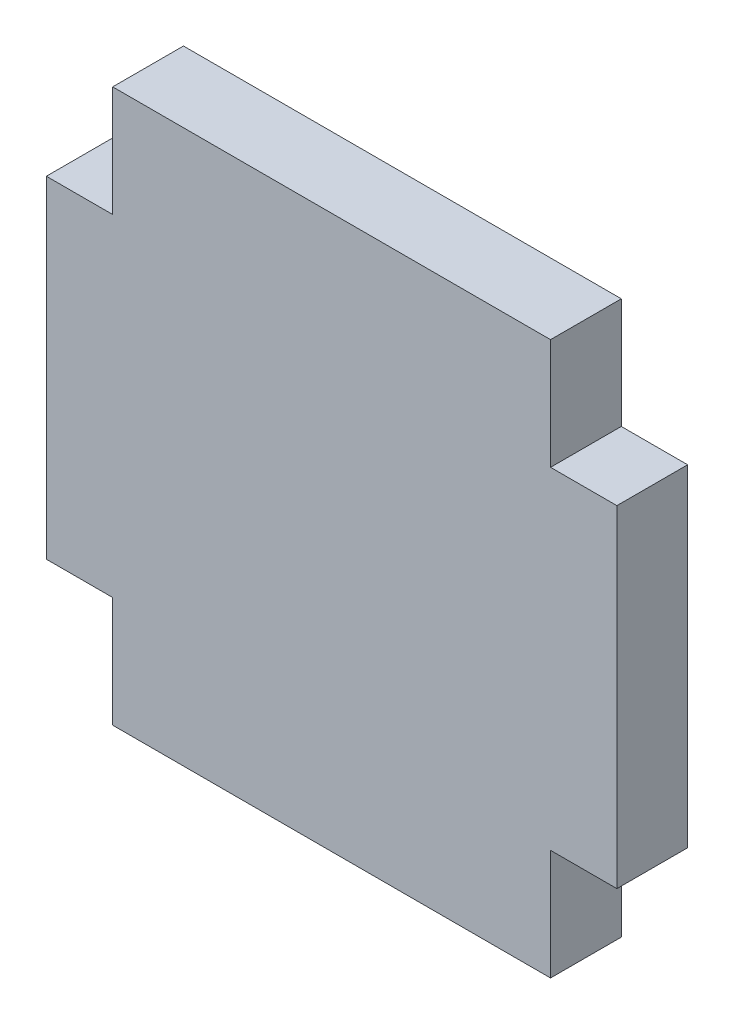
from build123d import *

# Parameters (mm, degrees)
BOSS_EXTRUDE1_DEPTH = 1.6


with BuildPart() as part:
    # Sketch1 → Boss-Extrude1 (new, symmetric)
    with BuildSketch(Plane.XY):
        Polygon((30.5, 25), (50.3, 25), (50.3, 30), (53.3, 30), (53.3, 45), (50.3, 45), (50.3, 50), (30.5, 50), (30.5, 45), (27.5, 45), (27.5, 30), (30.5, 30), align=None)
    extrude(amount=BOSS_EXTRUDE1_DEPTH, both=True)


solid = part.part
